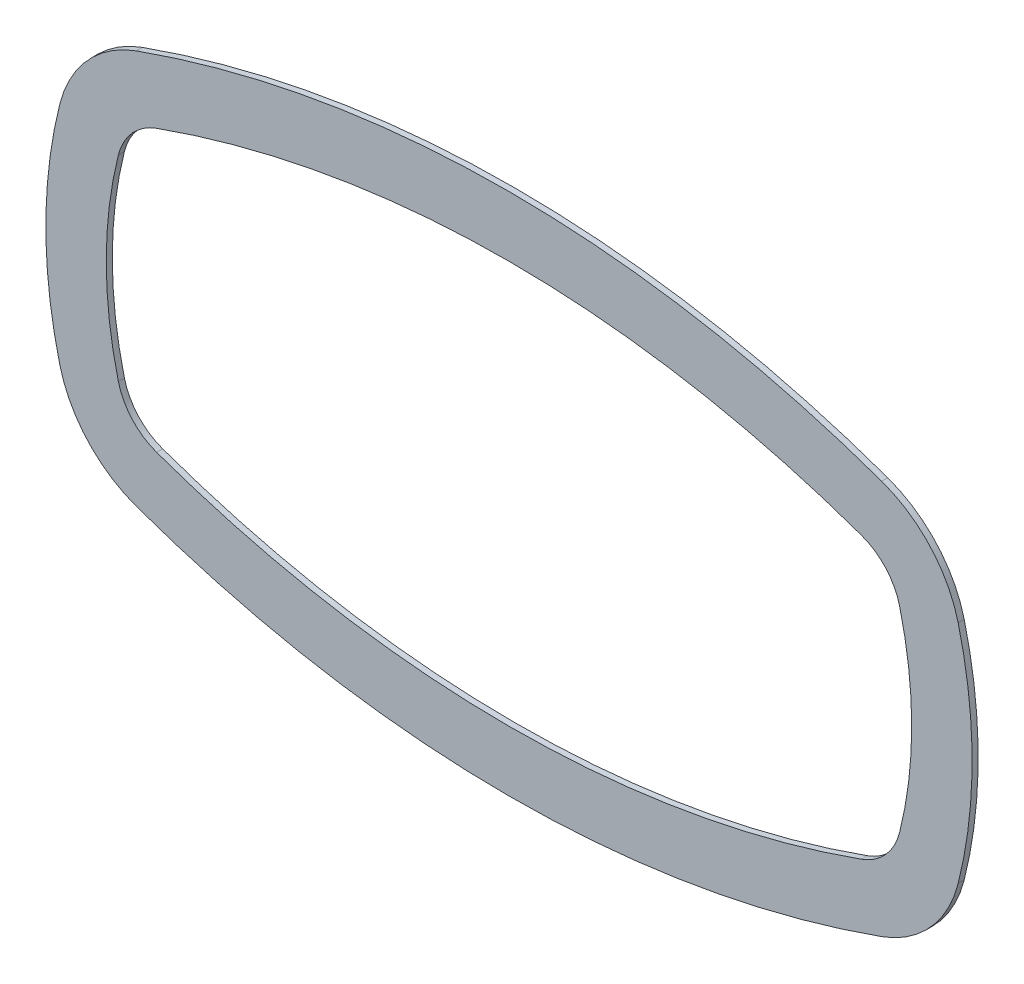
from build123d import *

# Parameters (mm, degrees)
BOSS_EXTRUDE1_DEPTH = 3


with BuildPart() as part:
    # Sketch1 → Boss-Extrude1 (new body)
    with BuildSketch(Plane.XY):
        with BuildLine():
            ThreePointArc((-185.063461818, 97.930029155), (0, 130), (185.063461818, 97.930029155))
            ThreePointArc((185.063461818, 97.930029155), (209.308091137, 81.748238793), (223.065798362, 56.050420168))
            ThreePointArc((223.065798362, 56.050420168), (230, 0), (223.065798362, -56.050420168))
            ThreePointArc((223.065798362, -56.050420168), (209.308091137, -81.748238793), (185.063461818, -97.930029155))
            ThreePointArc((185.063461818, -97.930029155), (0, -130), (-185.063461818, -97.930029155))
            ThreePointArc((-185.063461818, -97.930029155), (-209.308091137, -81.748238793), (-223.065798362, -56.050420168))
            ThreePointArc((-223.065798362, -56.050420168), (-230, 0), (-223.065798362, 56.050420168))
            ThreePointArc((-223.065798362, 56.050420168), (-209.308091137, 81.748238793), (-185.063461818, 97.930029155))
        make_face()
        with BuildLine():
            ThreePointArc((-174.969091173, 69.679300292), (0, 100), (174.969091173, 69.679300292))
            ThreePointArc((174.969091173, 69.679300292), (187.091405833, 61.588405111), (193.970259445, 48.739495798))
            ThreePointArc((193.970259445, 48.739495798), (200, 0), (193.970259445, -48.739495798))
            ThreePointArc((193.970259445, -48.739495798), (187.091405833, -61.588405111), (174.969091173, -69.679300292))
            ThreePointArc((174.969091173, -69.679300292), (0, -100), (-174.969091173, -69.679300292))
            ThreePointArc((-174.969091173, -69.679300292), (-187.091405833, -61.588405111), (-193.970259445, -48.739495798))
            ThreePointArc((-193.970259445, -48.739495798), (-200, 0), (-193.970259445, 48.739495798))
            ThreePointArc((-193.970259445, 48.739495798), (-187.091405833, 61.588405111), (-174.969091173, 69.679300292))
        make_face(mode=Mode.SUBTRACT)
    extrude(amount=BOSS_EXTRUDE1_DEPTH)


solid = part.part
